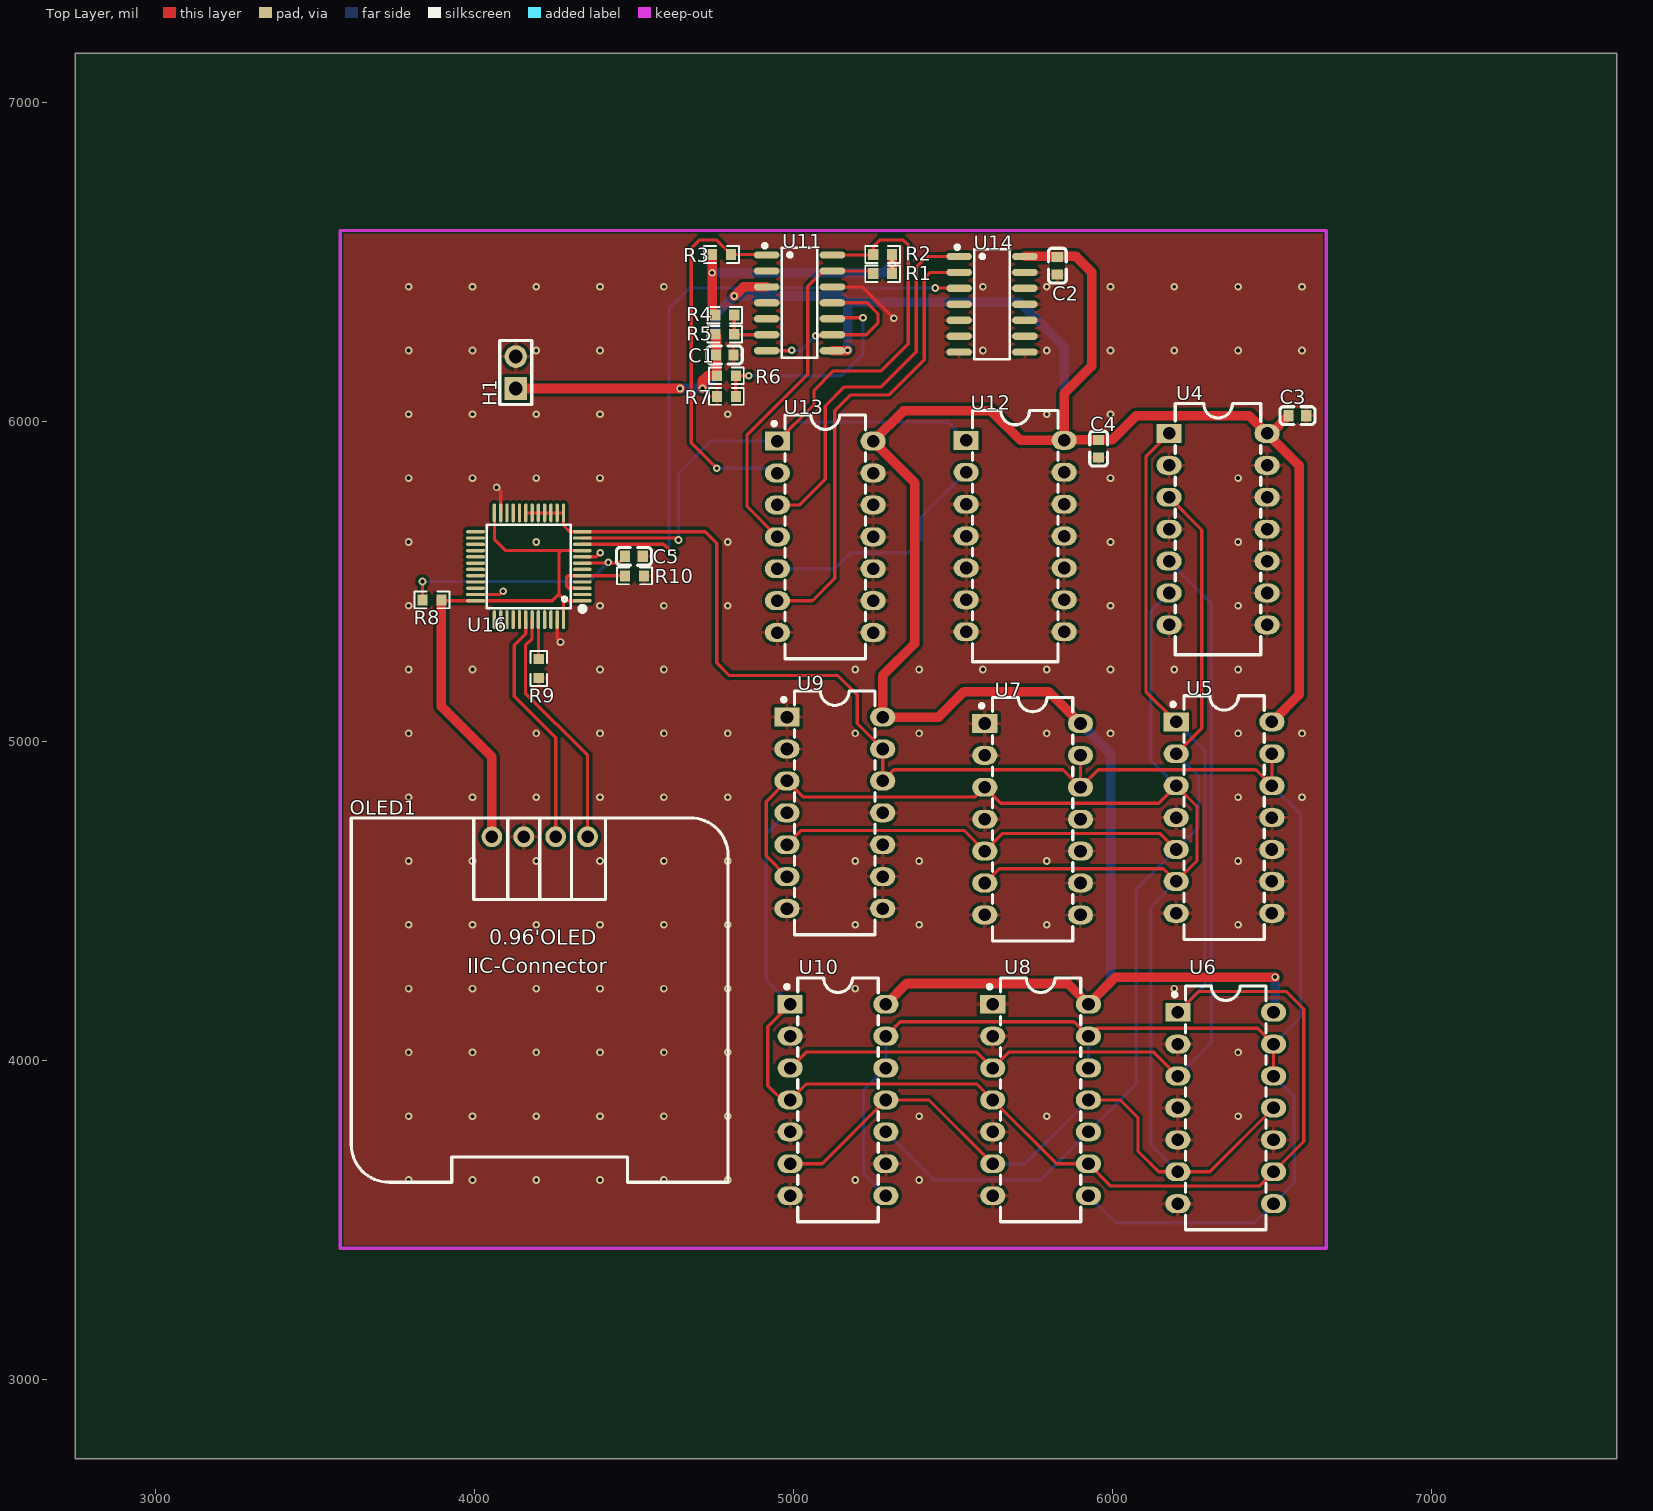
[diagram p0: Top Layer view]
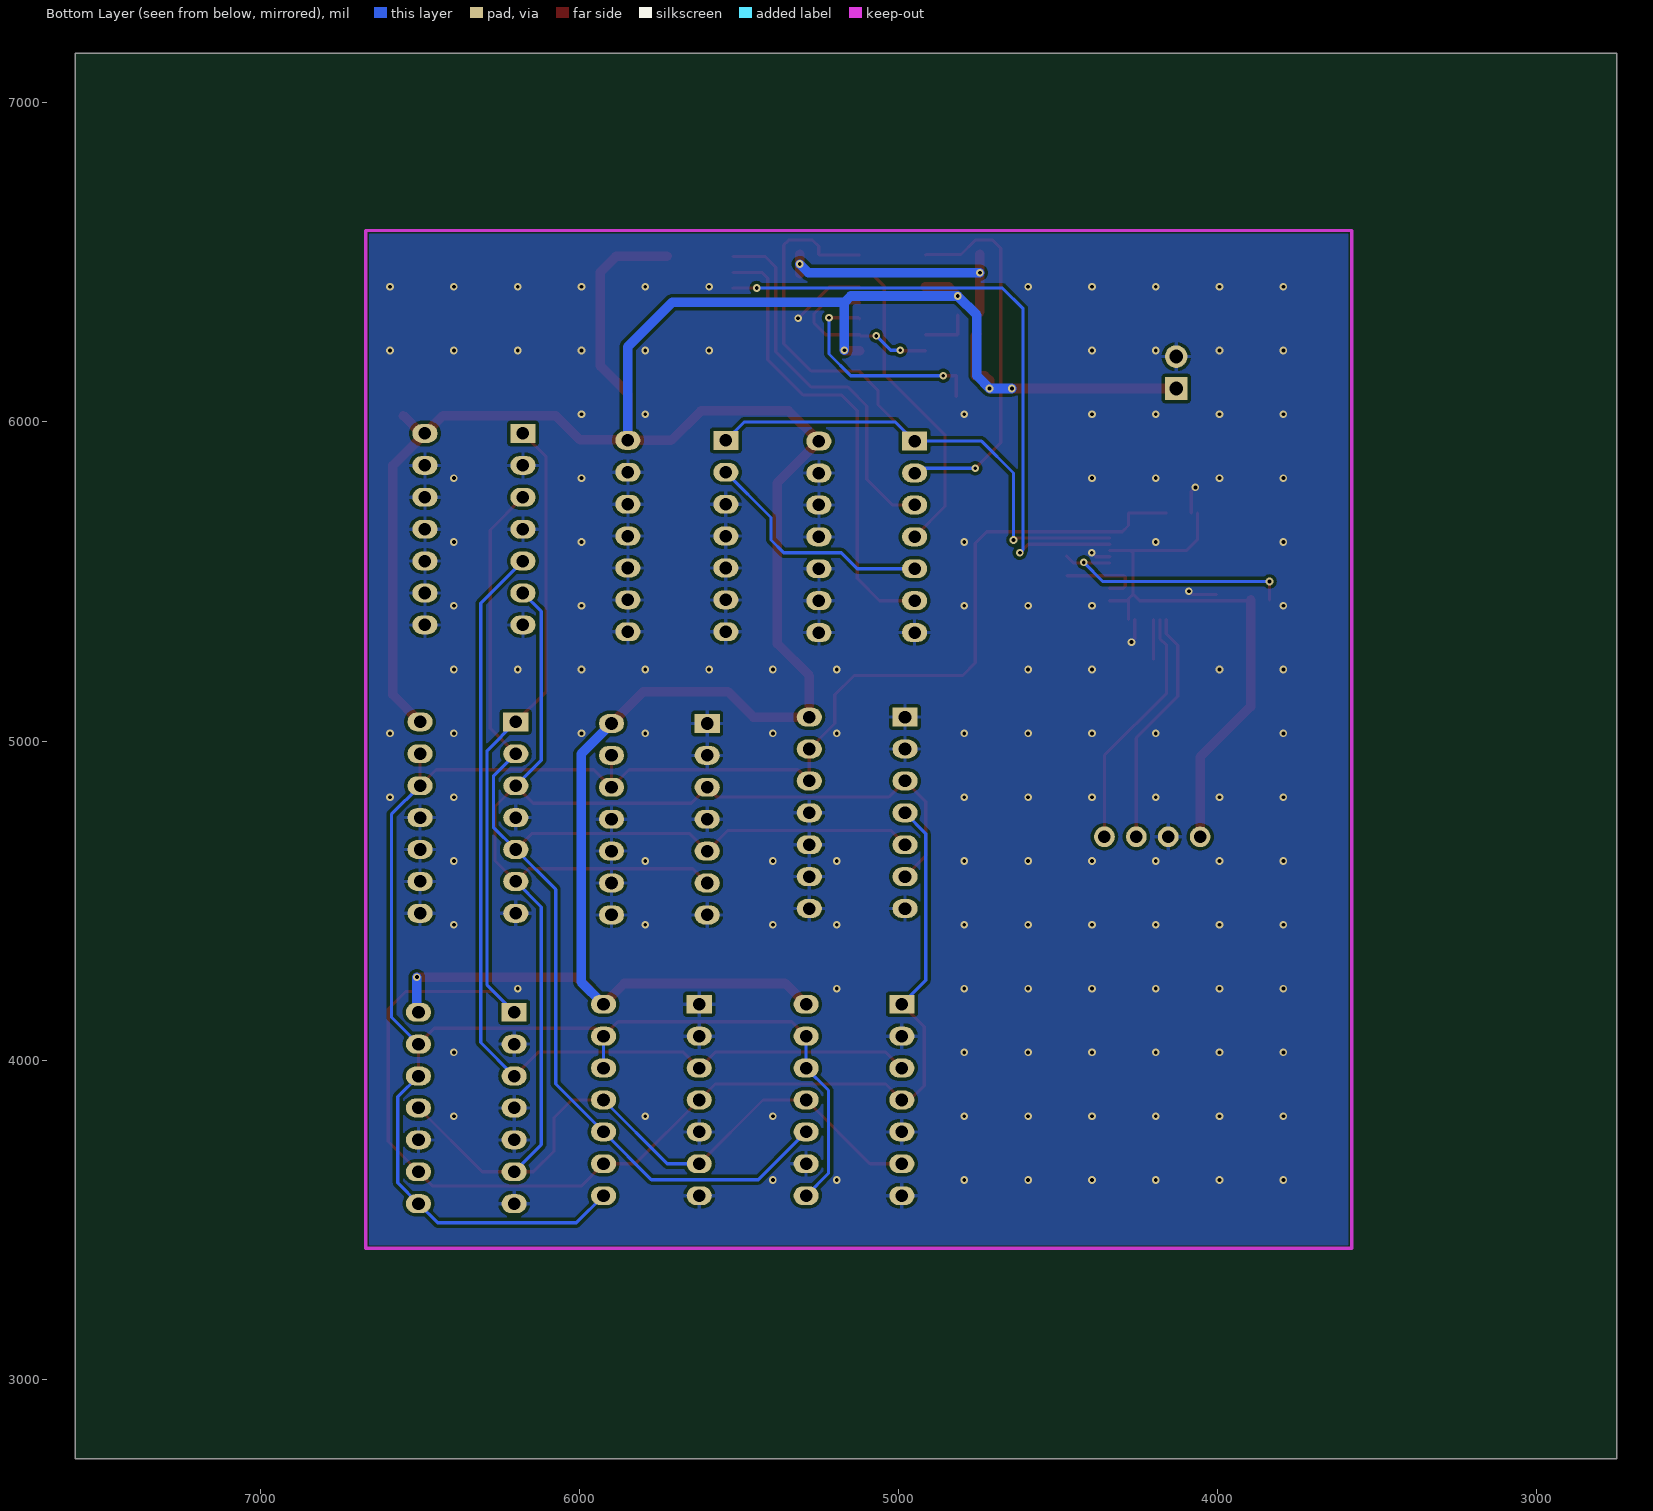
[diagram p1: Bottom Layer view, seen from below]
# Altium PCB MISC52068.pcbdoc
Units mil, origin at the board's own origin, x right, y up, seen from the top; angles counter-clockwise.
Board outline 4830 x 4405 mil, 2 copper layers (Top Layer, Bottom Layer), stack 62.206 mil thick; 29 components, 24 nets, 238 pads, 149 vias.

## Layer stack, top to bottom
Top Solder Mask Layer: solder mask 0.394, Dk 3.3
Top Layer: signal copper 1.379
Dielectric1: surface 59.449, FR4, Dk 4.5
Bottom Layer: signal copper 1.378
Bottom Solder Mask Layer: solder mask 0.394, Dk 3.3

## Board outline
7580,2750 2750,2750 2750,7155 7580,7155

## Design rules (kind name [scope] priority, off if disabled: settings)
BoardOutlineClearance copperThickness2oz_1 [All] p2 off: genericclearance=7.99 ignorepadtopadclearanceinfootprint=FALSE except(0: Arc-SplitContinuation Track-SplitContinuation SMDPad-SplitContinuation THPad-SplitContinuation Via-SplitContinuation Fill-SplitContinuation Region-SplitContinuation Poly-SplitContinuation Text-SplitContinuation Hole-SplitContinuation; 5.98: Arc-CutoutEdge SMDPad-CutoutEdge THPad-CutoutEdge Via-CutoutEdge Fill-CutoutEdge Region-CutoutEdge Text-CutoutEdge; 6.93: Hole-OutlineEdge Hole-CutoutEdge; 10: Poly-OutlineEdge Poly-CutoutEdge; 11.81: Arc-OutlineEdge Track-OutlineEdge SMDPad-OutlineEdge THPad-OutlineEdge Via-OutlineEdge Fill-OutlineEdge Region-OutlineEdge Text-OutlineEdge Track-CutoutEdge)
BoardOutlineClearance copperThickness1oz_1 [All] p4: genericclearance=4.02 ignorepadtopadclearanceinfootprint=FALSE except(0: Arc-SplitContinuation Track-SplitContinuation SMDPad-SplitContinuation THPad-SplitContinuation Via-SplitContinuation Fill-SplitContinuation Region-SplitContinuation Poly-SplitContinuation Text-SplitContinuation Hole-SplitContinuation; 6: SMDPad-CutoutEdge THPad-CutoutEdge Via-CutoutEdge Fill-CutoutEdge Region-CutoutEdge Text-CutoutEdge; 6.93: Hole-OutlineEdge Hole-CutoutEdge; 10: Poly-OutlineEdge Poly-CutoutEdge; 11.8: Arc-OutlineEdge Track-OutlineEdge SMDPad-OutlineEdge THPad-OutlineEdge Via-OutlineEdge Fill-OutlineEdge Region-OutlineEdge Text-OutlineEdge; 11.81: Arc-CutoutEdge Track-CutoutEdge)
Clearance copperThickness2oz [All] p1 off: gap=7.99 ignorepadtopadclearanceinfootprint=FALSE except(5.98: SMDPad-Track SMDPad-SMDPad THPad-Track SMDPad-THPad THPad-THPad Track-Via SMDPad-Via THPad-Via Via-Via Fill-Track Region-Track Fill-SMDPad Region-SMDPad Fill-THPad Region-THPad Fill-Via Region-Via Fill-Fill Fill-Region Region-Region Arc-Track Arc-SMDPad Arc-THPad Arc-Via Fill-Arc Region-Arc Arc-Arc Text-Track SMDPad-Text Text-THPad Text-Via Fill-Text Region-Text Arc-Text Text-Text; 6.93: Hole-Track Hole-SMDPad Hole-THPad Hole-Via Fill-Hole Region-Hole Hole-Arc Hole-Text; 10: Poly-Track Poly-SMDPad Poly-THPad Poly-Via Poly-Fill Poly-Region Poly-Poly Poly-Arc Poly-Text Poly-Hole)
Clearance copperThickness1oz [All] p3: gap=4.02 ignorepadtopadclearanceinfootprint=FALSE except(5.98: SMDPad-Track SMDPad-SMDPad THPad-Track SMDPad-THPad THPad-THPad Track-Via SMDPad-Via THPad-Via Via-Via Fill-Track Region-Track Fill-SMDPad Region-SMDPad Fill-THPad Region-THPad Fill-Via Region-Via Fill-Fill Fill-Region Region-Region; 6: Arc-Track Arc-SMDPad Arc-THPad Arc-Via Fill-Arc Region-Arc Arc-Arc Text-Track SMDPad-Text Text-THPad Text-Via Fill-Text Region-Text Arc-Text Text-Text; 6.93: Hole-Track Hole-SMDPad Hole-THPad Hole-Via Fill-Hole Region-Hole Hole-Arc Hole-Text; 10: Poly-Track Poly-SMDPad Poly-THPad Poly-Via Poly-Fill Poly-Region Poly-Poly Poly-Arc Poly-Text Poly-Hole)
DiffPairsRouting differentialPair [All] p1: maxlimit=6 minlimit=6 mostfreqgap=6 toplayer_minwidth=5 toplayer_prefwidth=10 toplayer_maxwidth=100 toplayer_mingap=6 toplayer_prefgap=6 toplayer_maxgap=6 bottomlayer_minwidth=5 bottomlayer_prefwidth=10 bottomlayer_maxwidth=100 bottomlayer_mingap=6 bottomlayer_prefgap=6 bottomlayer_maxgap=6 maxuncoupledlength=10
HoleToHoleClearance otherClearance [All] p1: gap=11.81 allowstackedmicrovias=TRUE
Length netLength [All] p1: minlimit=0 maxlimit=0
MatchedLengths netLengthTolerance [All] p1: tolerance=1000
PasteMaskExpansion pasteMaskExpansion [All] p1: expansion=0
PlaneConnect innerPlane [All] p1: planeconnectstyle=Relief reliefexpansion=20 reliefentries=4 reliefconductorwidth=10 reliefairgap=10
PolygonConnect copperRegion [(InNet('GND'))] p1: connectstyle=Relief reliefconductorwidth=10 reliefentries=4 polygonreliefangle="90 Angle" airgapwidth=10 via.connectstyle=Relief via.reliefconductorwidth=10 via.reliefentries=4 via.polygonreliefangle="90 Angle" via.airgapwidth=10
RoutingVias viaSize [All] p1: holewidth=12.01 width=24.02 viastyle="Through Hole" minholewidth=11.81 minwidth=19.68 maxholewidth=248.03 maxwidth=393.7
SolderMaskExpansion solderMaskExpansion [IsVia] p1: expansion=-1000 istentingtop=TRUE
SolderMaskExpansion solderMaskExpansion [All] p2: expansion=2 istentingtop=FALSE
Width copperThickness2oz_2 [All] p1 off: maxlimit=100 minlimit=8 preferedwidth=10
Width copperThickness1oz_2 [All] p2: maxlimit=100 minlimit=5 preferedwidth=10

## Components (designator, comment, footprint, x,y, rotation, side; value= is the part's Value field where it differs from the comment)
C1 "0.1u" C0603 4785,6210 r180 top
C2 "0.1u" C0603 5827.5,6489.97 r90 top
C3 "0.1u" C0603 6580,6020 r180 top
C4 "0.1u" C0603 5956.69,5916.49 r90 top
C5 "0.1u" C0603 4500.45,5579.13 r180 top
H1 "" HDR-TH_2P-P2.54-V-M-1 4130,6155 r90 top
OLED1 "0.96OLED_4P" 0.96OLED_4P 4205,4700 r0 top
R1 "10k" R0603 5280,6465 r180 top
R2 "1k" R0603 5280,6525 r0 top
R3 "1k" R0603 4775,6525 r180 top
R4 "2.2k" R0603 4785,6335 r180 top
R5 "2k" R0603 4785,6275 r0 top
R6 "100" R0603 4790,6145 r180 top
R7 "10" R0603 4790,6080 r0 top
R8 "10k" R0603 3867.14,5442.36 r180 top
R9 "10k" R0603 4202.14,5227.36 r90 top
R10 "10k" R0603 4502.14,5517.36 r180 top
U4 "74LS04DC" CDIP-14_L20.0-W6.8-P2.54-LS7.8-BL 6331.1,5664.05 r270 top
U5 "SN74LS11N" PDIP-14_L19.3-W6.4-P2.54-LS7.9-BL-1 6350,4760 r270 top
U6 "SN74LS11N" PDIP-14_L19.3-W6.4-P2.54-LS7.9-BL-1 6355,3850 r270 top
U7 "SN74LS11N" PDIP-14_L19.3-W6.4-P2.54-LS7.9-BL-1 5750,4755 r270 top
U8 "SN74LS11N" PDIP-14_L19.3-W6.4-P2.54-LS7.9-BL-1 5775,3875 r270 top
U9 "SN74LS11N" PDIP-14_L19.3-W6.4-P2.54-LS7.9-BL-1 5130,4775 r270 top
U10 "SN74LS11N" PDIP-14_L19.3-W6.4-P2.54-LS7.9-BL-1 5140,3875 r270 top
U11 "LM339D" SOIC-14_L8.7-W3.9-P1.27-LS6.0-BL 5019.35,6373.5 r270 top
U12 "74LS04DC" CDIP-14_L20.0-W6.8-P2.54-LS7.8-BL 5695.2,5642.4 r270 top
U13 "SN74LS08N" PDIP-14_L19.3-W6.4-P2.54-LS7.9-BL-1 5100,5640 r270 top
U14 "SN74LS32D" SOIC-14_L8.7-W3.9-P1.27-LS6.0-BL 5622.7,6368.99 r270 top
U16 "STM32F103C8T6" LQFP-48_L7.0-W7.0-P0.50-LS9.0-BL 4171.24,5547.83 r90 top

## Footprints (in the part's own frame and the unit in brackets; to place one, negate y for a bottom-side part, rotate by r counter-clockwise, add the part's x,y. Pads: shape width x height; smd on the part's side, far side on the other; paste and mask are expansions set on the pad)
0.96OLED_4P [mm]
  round 1.65 hole 1 copper offset 0,0: 1(-3.81,-0.001) 2(-1.27,0.002) 3(1.27,0.002) 4(3.81,0.002)
  silkscreen extent -15,-27.5 15,1.5
C0603 [mm]
  rect 0.8x0.9 smd: 1(-0.7,0) 2(0.7,0)
  silkscreen extent -1.39,-0.71 1.39,0.71
CDIP-14_L20.0-W6.8-P2.54-LS7.8-BL [mm]
  rect 1.5x2 hole 1: 1(-7.62,-3.9)
  oval 1.5x2 hole 1: 2(-5.08,-3.9) 3(-2.54,-3.9) 4(0,-3.9) 5(2.54,-3.9) 6(5.08,-3.9) 7(7.62,-3.9) 8(7.62,3.9) 9(5.08,3.9) 10(2.54,3.9) 11(0,3.9) 12(-2.54,3.9) 13(-5.08,3.9) 14(-7.62,3.9)
  silkscreen extent -10,-3.4 10,3.4
HDR-TH_2P-P2.54-V-M-1 [mm]
  rect 1.8x1.8 hole 1.1: 1(-1.27,0)
  round 1.8 hole 1.1: 2(1.27,0)
  silkscreen extent -2.54,-1.27 2.54,1.27
LQFP-48_L7.0-W7.0-P0.50-LS9.0-BL [mm]
  oval 0.27x1.5 smd paste+0 mask+0.05: 1(-2.75,-4.25) 2(-2.25,-4.25) 3(-1.75,-4.25) 4(-1.25,-4.25) 5(-0.75,-4.25) 6(-0.25,-4.25) 7(0.25,-4.25) 8(0.75,-4.25) 9(1.25,-4.25) 10(1.75,-4.25) 11(2.25,-4.25) 12(2.75,-4.25) 25(2.75,4.25) 26(2.25,4.25) 27(1.75,4.25) 28(1.25,4.25) 29(0.75,4.25) 30(0.25,4.25) 31(-0.25,4.25) 32(-0.75,4.25) 33(-1.25,4.25) 34(-1.75,4.25) 35(-2.25,4.25) 36(-2.75,4.25)
  oval 1.5x0.27 smd paste+0 mask+0.05: 13(4.25,-2.75) 14(4.25,-2.25) 15(4.25,-1.75) 16(4.25,-1.25) 17(4.25,-0.75) 18(4.25,-0.25) 19(4.25,0.25) 20(4.25,0.75) 21(4.25,1.25) 22(4.25,1.75) 23(4.25,2.25) 24(4.25,2.75) 37(-4.25,2.75) 38(-4.25,2.25) 39(-4.25,1.75) 40(-4.25,1.25) 41(-4.25,0.75) 42(-4.25,0.25) 43(-4.25,-0.25) 44(-4.25,-0.75) 45(-4.25,-1.25) 46(-4.25,-1.75) 47(-4.25,-2.25) 48(-4.25,-2.75)
  silkscreen extent -3.59,-4.46 3.3,3.34
PDIP-14_L19.3-W6.4-P2.54-LS7.9-BL-1 [mm]
  rect 1.5x2 hole 1: 1(-7.62,-3.81)
  oval 1.5x2 hole 1: 2(-5.08,-3.81) 3(-2.54,-3.81) 4(0,-3.81) 5(2.54,-3.81) 6(5.08,-3.81) 7(7.62,-3.81)
  oval 1.5x2 hole 1 copper offset 0,0: 8(7.62,3.81) 9(5.08,3.81) 10(2.54,3.81) 11(0,3.81) 12(-2.54,3.81) 13(-5.08,3.81) 14(-7.62,3.81)
  silkscreen extent -9.7,-4.21 9.7,3.2
R0603 [mil]
  rect 31.75x34.02 smd paste-3937.01 mask+2: 1(-29.66,0) 2(29.66,0)
  silkscreen extent -55,-26 55,26
SOIC-14_L8.7-W3.9-P1.27-LS6.0-BL [mil]
  oval 22.6x80.24 smd: 1(-150,-103.11) 2(-100,-103.11) 3(-50,-103.11) 4(0,-103.11) 5(50,-103.11) 6(100,-103.11) 7(150,-103.11) 8(150,103.11) 9(100,103.11) 10(50,103.11) 11(0,103.11) 12(-50,103.11) 13(-100,103.11) 14(-150,103.11)
  silkscreen extent -185,-115 172,55

## Via types
v1: diameter 24.02, hole 12, Top Layer to Bottom Layer, 149 vias

## Nets (pads, with @x,y where several pads share a name; then routed paths per layer and width w, separated by ;. In a path a pad name is that pad's centre, name@x,y a point inside that pad or via, vN(x,y) a via of type N, cw(c..) or ccw(c..) an arc to the next point about the centre after c; other vN are vias at no path point)
3.3V: OLED1.1 R8.1 U16.1 U16.9 U16.24 U16.36 U16.48 | length 1845.9
  Top Layer w10: R8.1 3899.6,5439.56 U16.36 4244.56,5439.56 4265,5460 ; U16.24 4062.97,5632.03 4097.93,5597.07 4272.07,5597.07 ; U16.48 4279.51,5445.49 ; U16.1 4285.44,5439.56 4279.51,5445.49 ; U16.9@4338.53,5597.07 4272.07,5597.07 ; 4265,5460 4265,5590 4272.07,5597.07 ; 4265,5460 4279.51,5445.49
  Top Layer w30: R8.1 3896.8,5108.2 4055,4950 OLED1.1
5V: R1.1 R2.2 R3.2 R4.2 | length 830.1
  Top Layer w30: R3.2 v1(4745.34,6467.69) 4745.34,6345 R4.2 ; R1.1 R2.2
  Bottom Layer w30: v1(4745.34,6467.69) 5282.69,6467.69 v1(5310,6495)
$3N1: R3.1 U11.1 U13.2 | length 1185.2
  Top Layer w10: v1(4760,5855) 4680,5935 4680,6545 4705,6570 4759.66,6570 R3.1 4914.74,6525 U11.1
  Bottom Layer w10: v1(4760,5855) 4935,5855 U13.2
$3N4: R4.1 R5.2 U11.6 | length 162.2
  Top Layer w10: R4.1 R5.2 4816.16,6273.5 U11.6
$3N6: R6.1 R7.2 U11.10 | length 702.5
  Top Layer w10: R7.2 R6.1 v1(4860,6145) ; U11.10 5125.69,6326.73 v1(5218.23,6326.73)
  Bottom Layer w10: v1(4860,6145) 5150,6145 5218.23,6213.23 v1(5218.23,6326.73)
$3N8: R1.2 U11.13 U13.4 | length 1132
  Top Layer w10: U13.4 4855,5735 4855,5960 5045,6150 5045,6425 5093.5,6473.5 U11.13 5241.84,6473.5 R1.2
$3N10: U12.2 U13.5 | length 758.4
  Bottom Layer w10: U13.5 5130,5540 5180,5590 5360,5590 5400,5630 5400,5700.74 U12.2
$3N11: U13.3 U14.1 | length 1182.2
  Top Layer w10: U13.3 5020,5740 5100,5820 5100,6050 5160,6110 5275,6110 5385,6220 5385,6485 5418.99,6518.99 U14.1
$3N12: U13.6 U14.2 | length 1452.7
  Top Layer w10: U13.6 5060,5440 5130,5510 5130,6035 5180,6085 5300,6085 5410,6195 5410,6450 5428.99,6468.99 U14.2
$4N2: R10.2 U16.3 U16.5 | length 265.3
  Top Layer w10: U16.3 4296.07,5478.93 4290,5485 4290,5515 4293.3,5518.3 U16.5 4471.54,5518.3 R10.2
$4N3: C5.2 R8.2 U16.7 | length 808.2
  Top Layer w10: R8.2 v1(3837.48,5500) ; U16.7 4451.43,5557.67 C5.2
  Bottom Layer w10: v1(3837.48,5500) 4360,5500 v1(4420,5560)
$4N15: OLED1.3 U16.42 | length 749.4
  Top Layer w10: U16.42 4161.4,5336.4 4125,5300 4125,5140 4255,5010 OLED1.3@4255,4700.05
$4N16: OLED1.4 U16.43 | length 770
  Top Layer w10: U16.43 4181.08,5321.08 4160,5300 4160,5150 4355,4955 OLED1.4@4355,4700.05
$4N17: R9.2 U16.44 | length 124.1
  Top Layer w10: U16.44 4200.77,5258.39 R9.2
A: U4.1 U5.1 U6.1 U6.9 U8.4 U8.9 U9.4 U10.1 U10.4 | length 5667.5
  Top Layer w10: U10.1 4920,4104.99 4920,3920 4965,3875 U10.4 5040,3925 5575,3925 U8.4 5825,3675 U8.9 5995,3605 6460,3605 U6.9 6600,3745 6600,4160 6545,4215 6270.01,4215 U6.1 ; U4.1 6105,5891.5 6105,5155.01 U5.1
  Bottom Layer w10: U9.4 4915,4710 4915,4250.01 U10.1 ; U5.1 6290,4970.01 6290,4234.99 U6.1
B: U4.3 U5.2 U5.5 U7.5 U8.10 U9.5 U10.10 | length 4304.8
  Top Layer w10: U9.5 5025,4720 5535,4720 U7.5 5655,4710 6150,4710 U5.5 ; U4.3 6280,5661.62 6280,5040 U5.2
  Bottom Layer w10: U10.10 5440,3625 5775,3625 U8.10 6075,3925 6075,4535 U5.5 6270,4730 6270,4890 U5.2
C: U4.5 U6.3 U8.3 U10.3 | length 3020.6
  Top Layer w10: U10.3 5040,4025 5575,4025 U8.3 5675,4025 6130,4025 U6.3
  Bottom Layer w10: U4.5 6310,5431.62 6310,4055 U6.3
C': U4.6 U5.3 U5.6 U6.6 U6.11 U7.3 U7.6 U8.6 U8.11 U9.3 U9.6 U10.6 U10.11 | length 6280
  Top Layer w10: U9.6 4915,4640 4915,4810 U9.3 5030,4825 5570,4825 U7.3 5650,4805 6145,4805 U5.3 6265,4795 6265,4625 U5.6 6160,4600 5645,4600 U7.6 ; U10.6 5090,3675 U10.11 5425,3875 U8.6 ; U8.11 6025,3875 6080,3820 6080,3715 6145,3650 U6.6 6305,3650 U6.11
  Bottom Layer w10: U8.6 5725,3675 U8.11 ; U4.6 6120,5406.49 6120,4940 U5.3 ; U5.6 6120,4480 6120,3735 U6.6
GND: C1.1 C2.1 C3.1 C4.1 C5.1 H1.2 OLED1.2 R7.1 R9.1 R10.1 U4.2 U4.4 U4.7 U4.8 U4.9 U4.10 U4.11 U4.12 U4.13 U5.4 U5.7 U5.8 U5.9 U5.10 U5.11 U6.2 U6.4 U6.5 U6.7 U6.10 U7.1 U7.2 U7.4 U7.7 U7.8 U7.9 U7.10 U7.11 U8.1 U8.2 U8.5 U8.7 U9.1 U9.2 U9.7 U9.8 U9.9 U9.10 U9.11 U10.2 U10.5 U10.7 U10.9 U11.2 U11.4 U11.5 U11.12 U12.3 U12.4 U12.5 U12.6 U12.7 U12.8 U12.9 U12.10 U12.11 U12.12 U12.13 U13.7 U13.8 U13.9 U13.10 U13.11 U13.12 U13.13 U14.4 U14.5 U14.6 U14.7 U14.8 U14.9 U14.10 U14.11 U14.12 U14.13 U16.8 U16.23 U16.35 U16.47 | length 545.6
  Top Layer w10: U16.35 4080,5459.25 v1(4090.38,5469.62) ; v1(4070,5795) 4082.66,5782.34 U16.23 ; U16.47 4259.82,5320.18 v1(4270,5310) ; U16.8 4382.36,5577.36 v1(4395,5590) ; U11.12 5216.5,6423.5 v1(5315,6325)
  other v1: 3794.1,3624.1 3994.1,3624.1 4194.1,3624.1 4394.1,3624.1 4594.1,3624.1 4794.1,3624.1 5194.1,3624.1 5394.1,3624.1 3794.1,3824.1 3994.1,3824.1 4194.1,3824.1 4394.1,3824.1 4594.1,3824.1 4794.1,3824.1 5394.1,3824.1 5794.1,3824.1 6394.1,3824.1 3794.1,4024.1 3994.1,4024.1 4194.1,4024.1 4394.1,4024.1 4594.1,4024.1 4794.1,4024.1 6394.1,4024.1 3794.1,4224.1 3994.1,4224.1 4194.1,4224.1 4394.1,4224.1 4594.1,4224.1 4794.1,4224.1 5194.1,4224.1 6194.1,4224.1 3794.1,4424.1 3994.1,4424.1 4194.1,4424.1 4394.1,4424.1 4594.1,4424.1 4794.1,4424.1 5194.1,4424.1 5394.1,4424.1 5794.1,4424.1 6394.1,4424.1 3794.1,4624.1 3994.1,4624.1 4194.1,4624.1 4394.1,4624.1 4594.1,4624.1 4794.1,4624.1 5194.1,4624.1 5394.1,4624.1 5794.1,4624.1 6394.1,4624.1 3794.1,4824.1 3994.1,4824.1 4194.1,4824.1 4394.1,4824.1 4594.1,4824.1 4794.1,4824.1 6394.1,4824.1 6594.1,4824.1 3794.1,5024.1 4194.1,5024.1 4394.1,5024.1 4594.1,5024.1 4794.1,5024.1 5194.1,5024.1 5394.1,5024.1 5794.1,5024.1 5994.1,5024.1 6394.1,5024.1 6594.1,5024.1 3794.1,5224.1 3994.1,5224.1 4394.1,5224.1 4594.1,5224.1 5194.1,5224.1 5394.1,5224.1 5594.1,5224.1 5794.1,5224.1 5994.1,5224.1 6194.1,5224.1 6394.1,5224.1 3794.1,5424.1 4394.1,5424.1 4594.1,5424.1 4794.1,5424.1 5994.1,5424.1 6394.1,5424.1 3794.1,5624.1 4194.1,5624.1 4794.1,5624.1 5994.1,5624.1 6394.1,5624.1 3794.1,5824.1 3994.1,5824.1 4194.1,5824.1 4394.1,5824.1 5994.1,5824.1 6394.1,5824.1 3794.1,6024.1 3994.1,6024.1 4194.1,6024.1 4394.1,6024.1 4794.1,6024.1 5794.1,6024.1 5994.1,6024.1 3794.1,6224.1 3994.1,6224.1 4194.1,6224.1 4394.1,6224.1 5594.1,6224.1 5794.1,6224.1 5994.1,6224.1 6194.1,6224.1 6394.1,6224.1 6594.1,6224.1 3794.1,6424.1 3994.1,6424.1 4194.1,6424.1 4394.1,6424.1 4594.1,6424.1 5594.1,6424.1 5794.1,6424.1 5994.1,6424.1 6194.1,6424.1 6394.1,6424.1 6594.1,6424.1
Q0: U14.3 U16.10 | length 1998.6
  Top Layer w10: U16.10 4593.27,5616.73 v1(4620,5590) ; v1(5445,6420) 5518.58,6420 U14.3
  Bottom Layer w10: v1(4620,5590) 4610,5600 4610,6355 4675,6420 v1(5445,6420)
Q1: R2.1 U11.14 U12.1 U13.1 U16.11 | length 2656.4
  Top Layer w10: U16.11 4633.59,5636.41 v1(4640,5630) ; U13.1 5065,6054.99 5065,6100 5125,6160 5275,6160 5360,6245 5360,6555 5345,6570 5270,6570 5250.34,6550.34 R2.1 5248.84,6523.5 U11.14
  Bottom Layer w10: v1(4640,5630) 4640,5840 4740,5940 U13.1 5010.01,6000 5484.05,6000 U12.1
VCC: C1.2 C2.2 C3.2 C4.2 H1.1 R5.1 R6.2 U4.14 U5.14 U6.14 U7.14 U8.14 U9.14 U10.14 U11.3 U11.8 U12.14 U13.14 U14.14 | length 10086.2
  Top Layer w30: H1.1 v1(4645,6105) ; v1(4715,6105) 4715,6130 4730,6145 R6.2 4760.34,6270 R5.1 ; v1(4815,6395) 4843.5,6423.5 U11.3 ; U11.8 5168.5,6223.5 v1(5170,6225) ; U10.14 5355,4240 5860,4240 U8.14 6010,4260 v1(6510,4260) ; U14.14 5886.01,6518.99 5935,6470 5935,6175 5848.74,6088.74 U12.14 ; U7.14 5800,5155 5535,5155 5455,5075 U9.14 5280,5205 5380,5305 5380,5810 U13.14 5345,6035 5620,6035 5712.6,5942.4 U12.14 ; U5.14 6585,5145 6585,5863.7 U4.14@6484.65,5964.05 ; C3.2 6496.49,5964.05 U4.14@6484.65,5964.05 ; U12.14 5850.39,5944.05 C4.2 5999.05,5944.05 6075,6020 6428.7,6020 U4.14@6484.65,5964.05
  Bottom Layer w30: v1(4645,6105) v1(4715,6105) 4755,6145 4755,6335 v1(4815,6395) 5150,6395 5170,6375 ; v1(5170,6225) 5170,6375 ; U12.14 5848.74,6236.26 5710,6375 5170,6375 ; U7.14 5995,4960 5995,4245 U8.14 ; U6.14 6510,4155 v1(6510,4260)
VIN: U11.7 U11.9 U11.11 | length 571
  Top Layer w10: U11.7 4993.5,6223.5 v1(4995,6225) ; v1(5070,6270) 5118.95,6270 U11.9 5228.5,6273.5 5265,6310 5265,6340 5231.5,6373.5 U11.11
  Bottom Layer w10: v1(4995,6225) 5025,6225 v1(5070,6270)
Y0: U5.12 U5.13 U6.8 U6.12 U6.13 U7.12 U7.13 U8.8 U8.12 U8.13 U9.12 U9.13 U10.8 U10.12 U10.13 U16.12 U16.13 U16.14 U16.15 U16.16 U16.17 U16.18 U16.19 | length 7339.3
  Top Layer w10: U16.19 U16.18 U16.17 U16.16 U16.15 U16.14 U16.13 4279.51,5675.49 4298.9,5656.1 U16.12 4723.9,5656.1 4760,5620 4760,5245 4800,5205 5140,5205 5200,5145 5200,5055 U9.13 U9.12 5315,4910 5845,4910 U7.12 ; U10.13 5335,4120 5880,4120 U8.13 5950,4100 6455,4100 U6.13 U6.12 ; U7.13 U7.12 ; U5.13 U5.12 6450,4910 5955,4910 U7.12
  Bottom Layer w10: U10.8 5220,3645 5220,3905 U10.12 U10.13 ; U8.8 6010,3490 6445,3490 U6.8 6570,3615 6570,3885 U6.12 ; U8.12 U8.13 ; U5.12 6590,4770 6590,4135 U6.13
pads on no net: U16.2 U16.4 U16.6 U16.20 U16.21 U16.22 U16.25 U16.26 U16.27 U16.28 U16.29 U16.30 U16.31 U16.32 U16.33 U16.34 U16.37 U16.38 U16.39 U16.40 U16.41 U16.45 U16.46

## Polygon pours and split planes (outlines as drawn)
GND on Bottom Layer (solid, remove dead copper, pour order 2): 3000,6905 3000,3000 7330,3000 7330,6905
GND on Top Layer (solid, remove dead copper, pour order 0): 3180,6860 3180,3380 7090,3380 7090,6860

## Keep-outs
Board Outline Layer:
  lines w10: 3580,3410 3580,6600 6670,6600 6670,3410 3580,3410